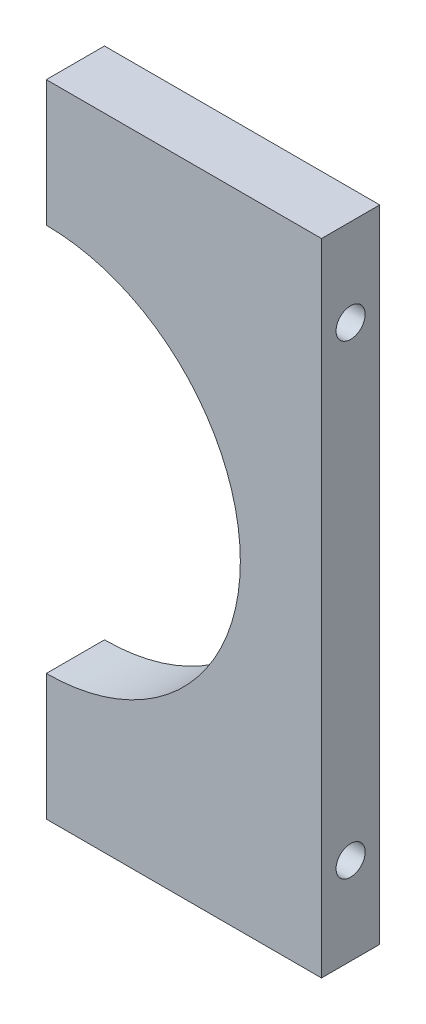
SolidWorks part; units mm, degrees
material "45"
ref_plane "Front Plane" through (0, 0, 0) normal (0, 0, 1) x (1, 0, 0)
ref_plane "Top Plane" through (0, 0, 0) normal (0, 1, 0) x (1, 0, 0)
ref_plane "Right Plane" through (0, 0, 0) normal (1, 0, 0) x (0, 0, -1)
sketch "Sketch2" plane through (0, 0, 0) normal (0, 0, 1) x (1, 0, 0)
  line L0 (16.5, -26.5041) -> (30.6825, -26.5041)
  line L1 (30.6825, -26.5041) -> (30.6825, 6.4959)
  line L2 (30.6825, 6.4959) -> (16.5, 6.4959)
  line L3 (16.5, 6.4959) -> (16.5, -0.0041)
  line L4 (16.5, -26.5041) -> (16.5, -20.0041)
  circle A0 centre (16.5, -10.0041) radius 10 construction
  arc A1 (16.5, -20.0041) -> (16.5, -0.0041) centre (16.5, -10.0041) ccw
extrude "Boss-Extrude1" add sketch "Sketch2" against normal blind 3
sketch "Sketch3" plane through (30.6825, 0, 0) normal (1, 0, 0) x (0, 0, -1)
  line L0 (3, -10.0041) -> (-11.1782, -10.0041) construction
  line L1 (3, -26.5041) -> (3, 6.4959) construction
  circle A0 centre (1.5, -22.0041) radius 0.75
  circle A1 centre (1.5, 1.9959) radius 0.75
  dimension "D1" = 1.5
  dimension "D2" = 12
extrude "Cut-Extrude1" cut sketch "Sketch3" against normal through all
